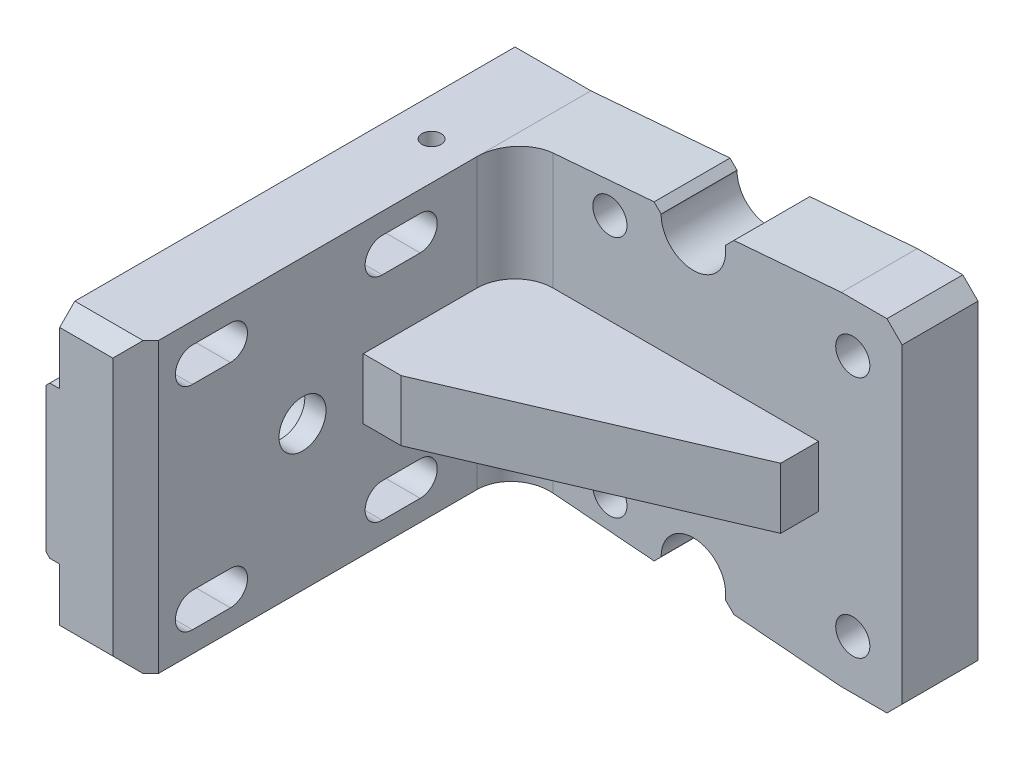
from build123d import *
from OCP.BRepFilletAPI import BRepFilletAPI_MakeChamfer

# Parameters (mm, degrees)
SKETCH1_W            = 61
SKETCH1_H            = 45
BOSS_EXTRUDE1_DEPTH  = 10
SKETCH2_W            = 10
SKETCH2_H            = 45
BOSS_EXTRUDE2_DEPTH  = 50
CUT_EXTRUDE3_DEPTH   = 82.897802168
SKETCH6_W            = 40
SKETCH6_H            = 8
BOSS_EXTRUDE3_DEPTH  = 20
CUT_EXTRUDE4_DEPTH   = 73.336021455
FILLET1_R            = 5
CUT_EXTRUDE5_DEPTH   = 71.968302784
LPATTERN2_COUNT      = 2
LPATTERN2_PITCH      = 28
LPATTERN2_COUNT_DIR2 = 2
LPATTERN2_PITCH_DIR2 = 25
SKETCH9_R            = 3
CUT_EXTRUDE6_DEPTH   = 5
SKETCH10_R           = 2.25
CUT_EXTRUDE7_DEPTH   = 71.968302784
CHAMFER1_SIZE        = 2
SKETCH4_W            = 60
SKETCH4_H            = 20
BOSS_EXTRUDE4_DEPTH  = 1.8
CHAMFER2_SIZE        = 0.5
SKETCH15_R           = 3.1
CUT_EXTRUDE8_DEPTH   = 82.897802168
SKETCH16_R           = 4.05
CUT_EXTRUDE9_DEPTH   = 9
CUT_EXTRUDE10_DEPTH  = 10
CHAMFER3_SIZE        = 1
CHAMFER3_SIZE2       = 0.927789392
CHAMFER3_SIZE2_2     = 1.092207765
CHAMFER4_SIZE        = 3


with BuildPart() as part:
    # Sketch1 → Boss-Extrude1 (new body)
    with BuildSketch(Plane.XY):
        Rectangle(SKETCH1_W, SKETCH1_H)
    extrude(amount=BOSS_EXTRUDE1_DEPTH)

    # Sketch2 → Boss-Extrude2 (add)
    with BuildSketch(Plane.XY.offset(10)):
        with Locations((-25.5, 0)):
            Rectangle(SKETCH2_W, SKETCH2_H)
    extrude(amount=BOSS_EXTRUDE2_DEPTH)

    # Sketch5 → Cut-Extrude3 (cut, through all)
    with BuildSketch(Plane(origin=(-20.5, 0, 0), x_dir=(0, 0, -1), z_dir=(1, 0, 0))):
        with BuildLine():
            Line((-52.5, -11.75), (-47.5, -11.75))
            ThreePointArc((-47.5, -11.75), (-45.25, -14), (-47.5, -16.25))
            Line((-47.5, -16.25), (-52.5, -16.25))
            ThreePointArc((-52.5, -16.25), (-54.75, -14), (-52.5, -11.75))
        make_face()
    cut_extrude3 = extrude(amount=-CUT_EXTRUDE3_DEPTH, mode=Mode.SUBTRACT)

    # Sketch6 → Boss-Extrude3 (add)
    with BuildSketch(Plane.XY.offset(10)):
        with Locations((-0.5, 0)):
            Rectangle(SKETCH6_W, SKETCH6_H)
    extrude(amount=BOSS_EXTRUDE3_DEPTH)

    # Sketch7 → Cut-Extrude4 (cut, through all)
    with BuildSketch(Plane.XZ.offset(4)):
        Polygon((19.5, 30), (-15.5, 30), (19.5, 15), align=None)
    extrude(amount=-CUT_EXTRUDE4_DEPTH, mode=Mode.SUBTRACT)

    # Fillet1
    fillet1_edges = [part.edges().sort_by_distance(p)[0] for p in [
        (-20.5, 13.25, 10),
        (-20.5, -13.25, 10),
    ]]
    fillet(fillet1_edges, radius=FILLET1_R)

    # Sketch8 → Cut-Extrude5 (cut, through all)
    with BuildSketch(Plane.XY.offset(60)):
        Polygon((-30.5, 22.5), (22.5, 22.5), (-20.5, 19), (-30.5, 19), align=None)
        Polygon((-20.5, -19), (22.5, -22.5), (-30.5, -22.5), (-30.5, -19), align=None)
    extrude(amount=-CUT_EXTRUDE5_DEPTH, mode=Mode.SUBTRACT)

    # LPattern2: Cut-Extrude3 2 × 2
    with Locations(*[(0, i * LPATTERN2_PITCH, -j * LPATTERN2_PITCH_DIR2) for i in range(LPATTERN2_COUNT) for j in range(LPATTERN2_COUNT_DIR2) if (i, j) != (0, 0)]):
        add(cut_extrude3, mode=Mode.SUBTRACT)

    # Sketch9 → Cut-Extrude6 (cut)
    with BuildSketch(Plane(origin=(0, 0, 0), x_dir=(-1, 0, 0), z_dir=(0, 0, -1))):
        with Locations((-25, 0)):
            Circle(SKETCH9_R)
        with BuildLine():
            Line((8.75, -3), (7.25, -3))
            ThreePointArc((7.25, -3), (4.25, 0), (7.25, 3))
            Line((7.25, 3), (8.75, 3))
            ThreePointArc((8.75, 3), (11.75, 0), (8.75, -3))
        make_face()
    extrude(amount=-CUT_EXTRUDE6_DEPTH, mode=Mode.SUBTRACT)

    # Sketch10 → Cut-Extrude7 (cut, through all)
    with BuildSketch(Plane(origin=(0, 0, 0), x_dir=(-1, 0, 0), z_dir=(0, 0, -1))):
        with Locations((8, -16)):
            Circle(SKETCH10_R)
        with Locations((-24, -16)):
            Circle(SKETCH10_R)
        with Locations((-24, 16)):
            Circle(SKETCH10_R)
        with Locations((8, 16)):
            Circle(SKETCH10_R)
    extrude(amount=-CUT_EXTRUDE7_DEPTH, mode=Mode.SUBTRACT)

    # Chamfer1
    chamfer1_edges = [part.edges().sort_by_distance(p)[0] for p in [
        (30.5, -22.5, 5),
        (30.5, 22.5, 5),
        (-25.5, -19, 60),
        (-25.5, 19, 60),
    ]]
    chamfer(chamfer1_edges, length=CHAMFER1_SIZE)

    # Sketch13 → M3 Tapped Hole1 (revolve, cut)
    with BuildSketch(Plane(origin=(-25.5, 19, 16), x_dir=(0, 0, 1), z_dir=(1, 0, 0))):
        Polygon((0, 0), (0, 8.251075774), (1.25, 7.5), (1.25, 0), align=None)
    m3_tapped_hole1 = revolve(axis=Axis((-25.5, 25.35, 16), (0, -1, 0)), mode=Mode.SUBTRACT)

    # Mirror1: M3 Tapped Hole1 across plane
    add(m3_tapped_hole1.mirror(Plane.ZX), mode=Mode.SUBTRACT)

    # Sketch4 → Boss-Extrude4 (add)
    with BuildSketch(Plane.ZY.offset(30.5)):
        with Locations((30, 0)):
            Rectangle(SKETCH4_W, SKETCH4_H)
    extrude(amount=BOSS_EXTRUDE4_DEPTH)

    # Chamfer2
    chamfer2_edges = [part.edges().sort_by_distance(p)[0] for p in [
        (-32.3, 10, 30),
        (-32.3, -10, 30),
    ]]
    chamfer(chamfer2_edges, length=CHAMFER2_SIZE)

    # Sketch15 → Cut-Extrude8 (cut, through all)
    with BuildSketch(Plane(origin=(-20.5, 0, 0), x_dir=(0, 0, -1), z_dir=(1, 0, 0))):
        with Locations(Location((-38, 0, 0), (0, 0, 90))):
            Circle(SKETCH15_R)
    extrude(amount=-CUT_EXTRUDE8_DEPTH, mode=Mode.SUBTRACT)

    # Sketch16 → Cut-Extrude9 (cut)
    with BuildSketch(Plane.ZY.offset(32.3)):
        with Locations((38, 0)):
            Circle(SKETCH16_R)
    extrude(amount=-CUT_EXTRUDE9_DEPTH, mode=Mode.SUBTRACT)

    # Sketch17 → Cut-Extrude10 (cut)
    with BuildSketch(Plane.XY.offset(10)):
        with BuildLine():
            Line((7.25, -19.5), (7.25, -28.943782823))
            ThreePointArc((7.25, -28.943782823), (3, -33.193782823), (-1.25, -28.943782823))
            Line((-1.25, -28.943782823), (-1.25, -19.5))
            ThreePointArc((-1.25, -19.5), (3, -15.25), (7.25, -19.5))
        make_face()
        with BuildLine():
            Line((-1.25, 19.5), (-1.25, 28.943782823))
            ThreePointArc((-1.25, 28.943782823), (3, 33.193782823), (7.25, 28.943782823))
            Line((7.25, 28.943782823), (7.25, 19.5))
            ThreePointArc((7.25, 19.5), (3, 15.25), (-1.25, 19.5))
        make_face()
    extrude(amount=-CUT_EXTRUDE10_DEPTH, mode=Mode.SUBTRACT)

    # Chamfer3: one chamfer whose edges measure the first distance from different faces: ONE call of the kernel's chamfer builder (chamfer() names one face for all edges)
    chamfer3_edges_1 = [part.edges().sort_by_distance(p)[0] for p in [
        (-1.25, -20.566860465, 5),
    ]]
    chamfer3_side_1 = [part.faces().sort_by_distance(p)[0] for p in [
        (-1.25, -20.033430233, 5),
    ]]
    chamfer3_edges_2 = [part.edges().sort_by_distance(p)[0] for p in [
        (7.25, -21.25872093, 5),
    ]]
    chamfer3_side_2 = [part.faces().sort_by_distance(p)[0] for p in [
        (7.25, -20.379360465, 5),
    ]]
    chamfer3_edges_3 = [part.edges().sort_by_distance(p)[0] for p in [
        (7.25, 21.25872093, 5),
    ]]
    chamfer3_side_3 = [part.faces().sort_by_distance(p)[0] for p in [
        (7.25, 20.379360465, 5),
    ]]
    chamfer3_edges_4 = [part.edges().sort_by_distance(p)[0] for p in [
        (-1.25, 20.566860465, 5),
    ]]
    chamfer3_side_4 = [part.faces().sort_by_distance(p)[0] for p in [
        (-1.25, 20.033430233, 5),
    ]]
    chamfer3 = BRepFilletAPI_MakeChamfer(part.part.solid().wrapped)
    for e in chamfer3_edges_1:
        chamfer3.Add(CHAMFER3_SIZE, CHAMFER3_SIZE2, e.wrapped, chamfer3_side_1[0].wrapped)  # the first distance lies on this face
    for e in chamfer3_edges_2:
        chamfer3.Add(CHAMFER3_SIZE, CHAMFER3_SIZE2_2, e.wrapped, chamfer3_side_2[0].wrapped)  # the first distance lies on this face
    for e in chamfer3_edges_3:
        chamfer3.Add(CHAMFER3_SIZE, CHAMFER3_SIZE2_2, e.wrapped, chamfer3_side_3[0].wrapped)  # the first distance lies on this face
    for e in chamfer3_edges_4:
        chamfer3.Add(CHAMFER3_SIZE, CHAMFER3_SIZE2, e.wrapped, chamfer3_side_4[0].wrapped)  # the first distance lies on this face
    add(Compound.cast(chamfer3.Shape()), mode=Mode.REPLACE)

    # Chamfer4
    chamfer4_edges = [part.edges().sort_by_distance(p)[0] for p in [
        (-20.5, 0, 60),
    ]]
    chamfer(chamfer4_edges, length=CHAMFER4_SIZE)


solid = part.part
